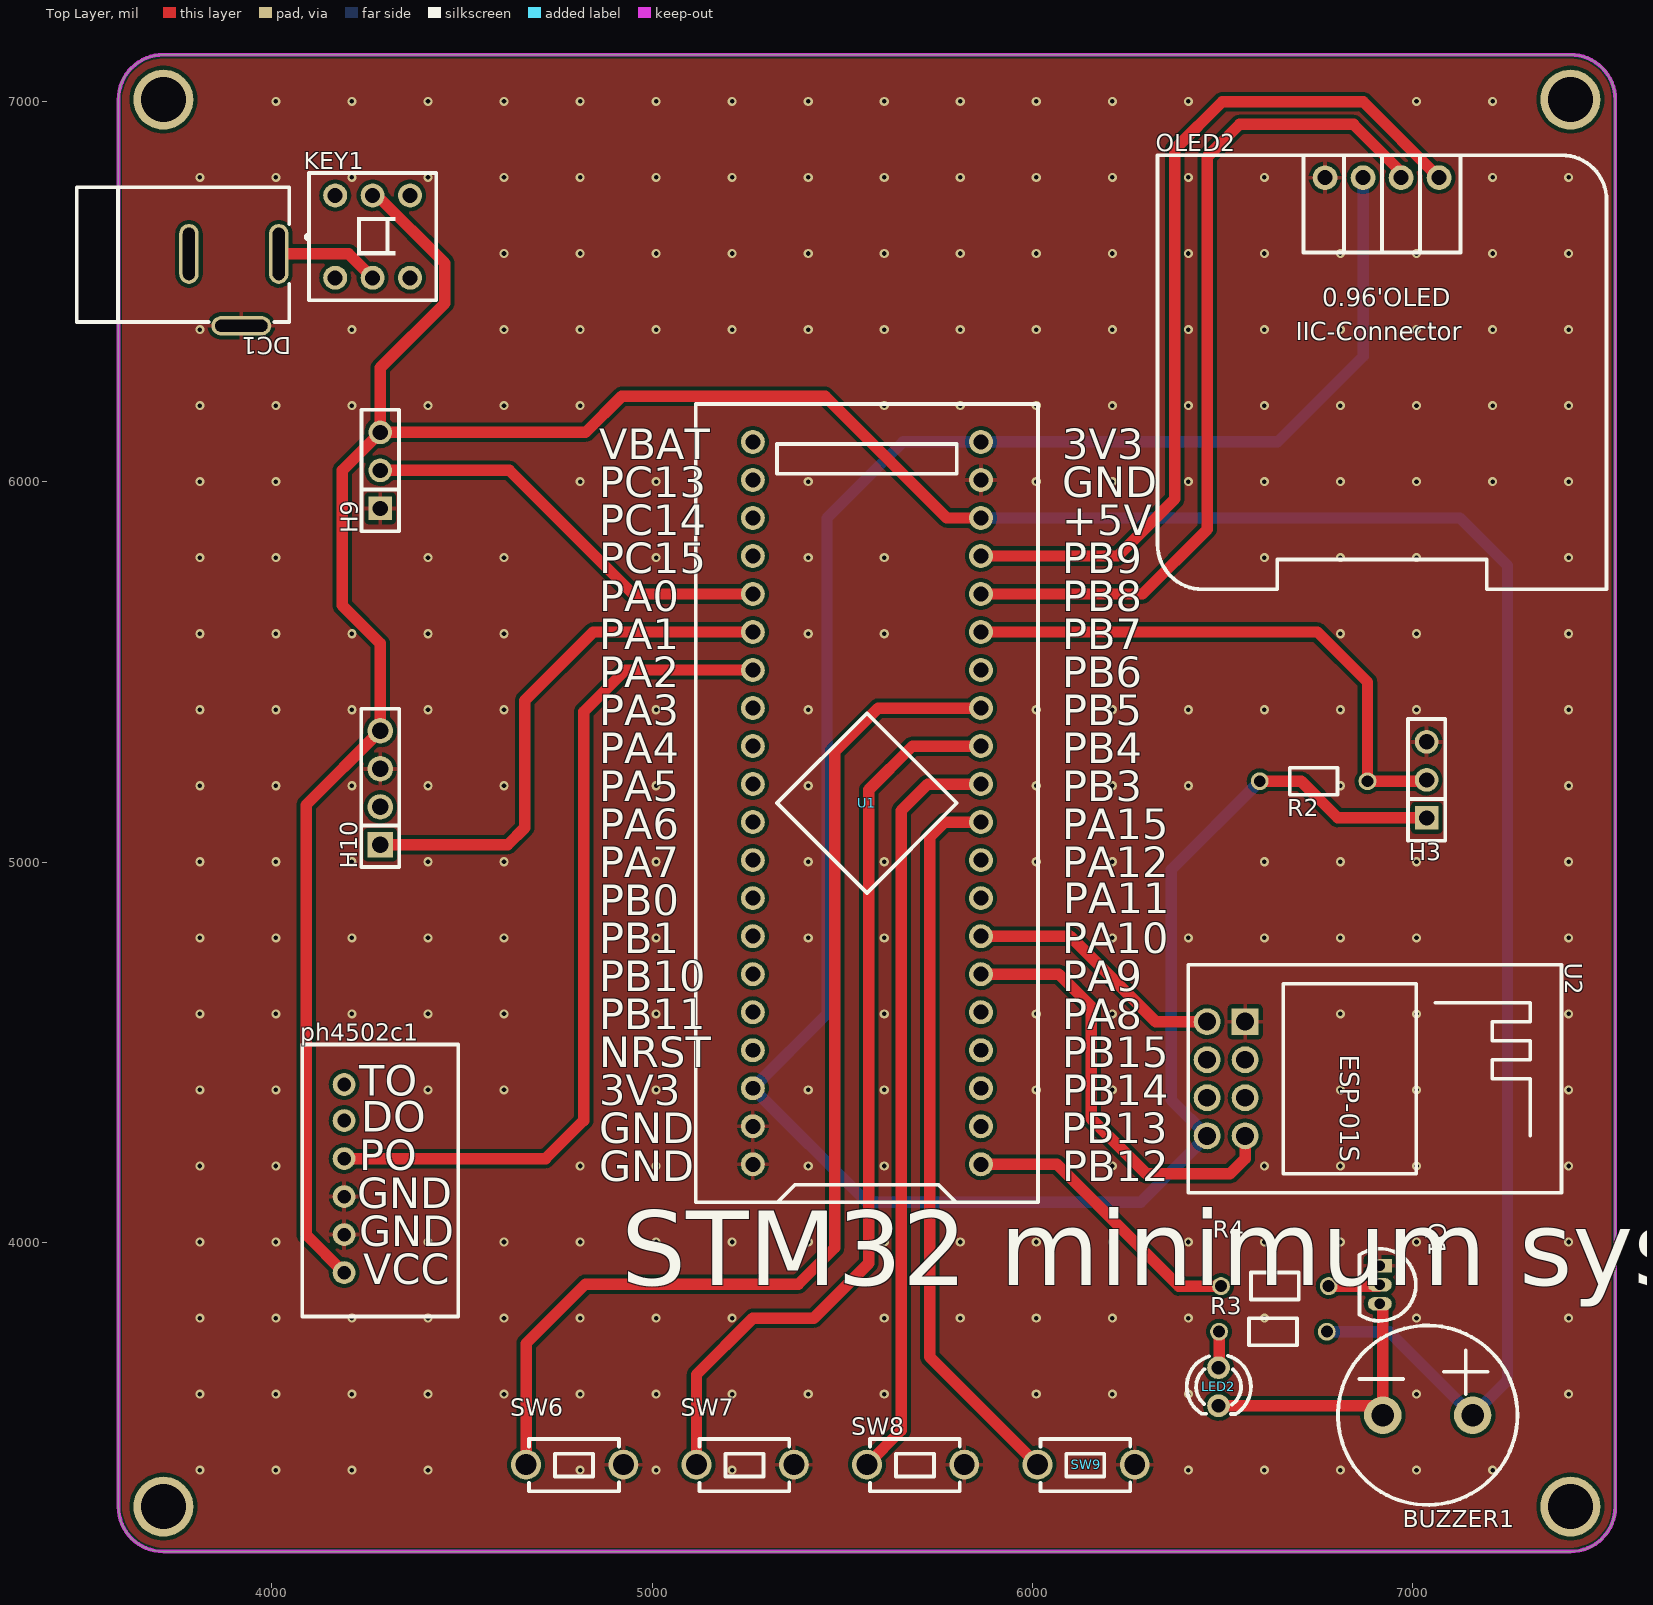
[diagram p0: Top Layer view]
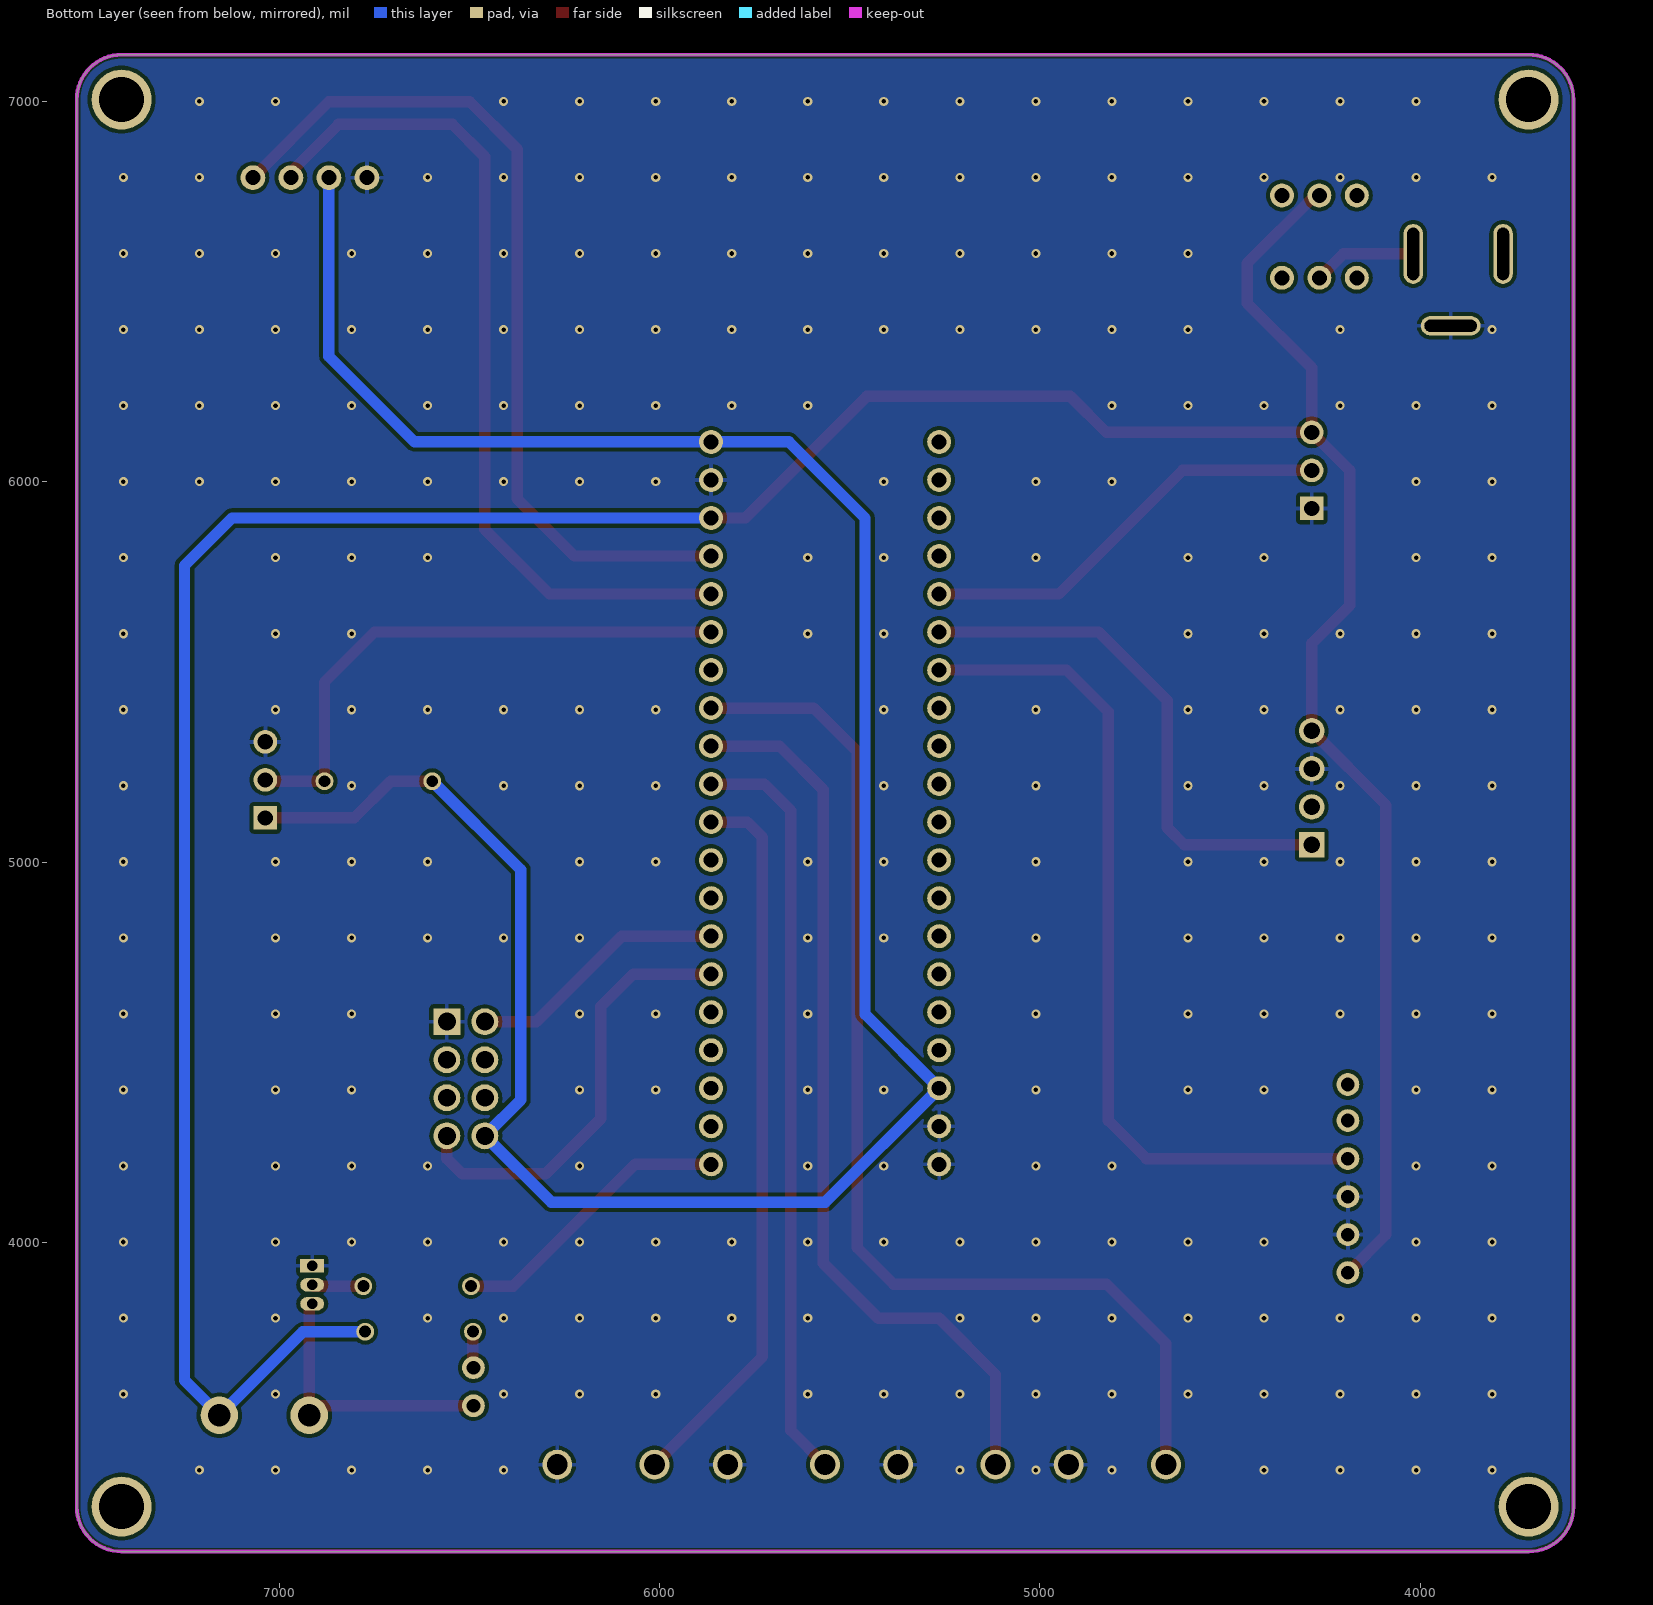
[diagram p1: Bottom Layer view, seen from below]
# Altium PCB MISC49912.pcbdoc
Units mil, origin at the board's own origin, x right, y up, seen from the top; angles counter-clockwise.
Board outline 3937.01 x 3937.01 mil, 2 copper layers (Top Layer, Bottom Layer), stack 62.206 mil thick; 19 components, 41 nets, 102 pads, 263 vias.

## Layer stack, top to bottom
Top Solder Mask Layer: solder mask 0.394, Dk 3.3
Top Layer: signal copper 1.379
Dielectric1: surface 59.449, FR4, Dk 4.5
Bottom Layer: signal copper 1.378
Bottom Solder Mask Layer: solder mask 0.394, Dk 3.3

## Board outline
3714.61,7123.5 ccw(c3714.61,7005.39) 3596.5,7005.39 3596.5,3304.61 ccw(c3714.61,3304.61) 3714.61,3186.5 7415.39,3186.5 ccw(c7415.39,3304.61) 7533.5,3304.61 7533.5,7005.39 ccw(c7415.39,7005.39) 7415.39,7123.5 3714.61,7123.5

## Design rules (kind name [scope] priority, off if disabled: settings)
BoardOutlineClearance copperThickness2oz_1 [All] p2 off: genericclearance=7.99 ignorepadtopadclearanceinfootprint=FALSE except(0: Arc-SplitContinuation Track-SplitContinuation SMDPad-SplitContinuation THPad-SplitContinuation Via-SplitContinuation Fill-SplitContinuation Region-SplitContinuation Poly-SplitContinuation Text-SplitContinuation Hole-SplitContinuation; 5.98: Arc-CutoutEdge Track-CutoutEdge SMDPad-CutoutEdge THPad-CutoutEdge Via-CutoutEdge Text-CutoutEdge; 6.9: Hole-OutlineEdge Hole-CutoutEdge; 10: Poly-OutlineEdge Poly-CutoutEdge; 11.81: Arc-OutlineEdge Track-OutlineEdge SMDPad-OutlineEdge THPad-OutlineEdge Via-OutlineEdge Fill-OutlineEdge Region-OutlineEdge Text-OutlineEdge Fill-CutoutEdge Region-CutoutEdge)
BoardOutlineClearance Plane_innerPlane_1 [All] p4 off: genericclearance=4.02 ignorepadtopadclearanceinfootprint=FALSE except(0: Arc-SplitContinuation Track-SplitContinuation SMDPad-SplitContinuation THPad-SplitContinuation Via-SplitContinuation Fill-SplitContinuation Region-SplitContinuation Poly-SplitContinuation Text-SplitContinuation Hole-SplitContinuation; 5.98: Arc-CutoutEdge Track-CutoutEdge SMDPad-CutoutEdge THPad-CutoutEdge Via-CutoutEdge Text-CutoutEdge; 6.9: Hole-OutlineEdge Hole-CutoutEdge; 10: Poly-OutlineEdge Poly-CutoutEdge; 11.81: Arc-OutlineEdge Track-OutlineEdge SMDPad-OutlineEdge THPad-OutlineEdge Via-OutlineEdge Fill-OutlineEdge Region-OutlineEdge Text-OutlineEdge Fill-CutoutEdge Region-CutoutEdge)
BoardOutlineClearance Copper_copperRegion_1 [All] p6 off: genericclearance=4.02 ignorepadtopadclearanceinfootprint=FALSE except(0: Arc-SplitContinuation Track-SplitContinuation SMDPad-SplitContinuation THPad-SplitContinuation Via-SplitContinuation Fill-SplitContinuation Region-SplitContinuation Poly-SplitContinuation Text-SplitContinuation Hole-SplitContinuation; 5.98: Arc-CutoutEdge Track-CutoutEdge SMDPad-CutoutEdge THPad-CutoutEdge Via-CutoutEdge Text-CutoutEdge; 6.9: Hole-OutlineEdge Hole-CutoutEdge; 10: Poly-OutlineEdge Poly-CutoutEdge; 11.81: Arc-OutlineEdge Track-OutlineEdge SMDPad-OutlineEdge THPad-OutlineEdge Via-OutlineEdge Fill-OutlineEdge Region-OutlineEdge Text-OutlineEdge Fill-CutoutEdge Region-CutoutEdge)
BoardOutlineClearance Copper_copperRegion_copperThickness1oz_1 [All] p8 off: genericclearance=4.02 ignorepadtopadclearanceinfootprint=FALSE except(0: Arc-SplitContinuation Track-SplitContinuation SMDPad-SplitContinuation THPad-SplitContinuation Via-SplitContinuation Fill-SplitContinuation Region-SplitContinuation Poly-SplitContinuation Text-SplitContinuation Hole-SplitContinuation; 5.98: Arc-CutoutEdge Track-CutoutEdge SMDPad-CutoutEdge THPad-CutoutEdge Via-CutoutEdge Text-CutoutEdge; 6.9: Hole-OutlineEdge Hole-CutoutEdge; 10: Poly-OutlineEdge Poly-CutoutEdge; 11.81: Arc-OutlineEdge Track-OutlineEdge SMDPad-OutlineEdge THPad-OutlineEdge Via-OutlineEdge Fill-OutlineEdge Region-OutlineEdge Text-OutlineEdge Fill-CutoutEdge Region-CutoutEdge)
BoardOutlineClearance Copper_copperRegion_Copper_copperRegion_1 [All] p10 off: genericclearance=4.02 ignorepadtopadclearanceinfootprint=FALSE except(0: Arc-SplitContinuation Track-SplitContinuation SMDPad-SplitContinuation THPad-SplitContinuation Via-SplitContinuation Fill-SplitContinuation Region-SplitContinuation Poly-SplitContinuation Text-SplitContinuation Hole-SplitContinuation; 5.98: Arc-CutoutEdge Track-CutoutEdge SMDPad-CutoutEdge THPad-CutoutEdge Via-CutoutEdge Text-CutoutEdge; 6.9: Hole-OutlineEdge Hole-CutoutEdge; 10: Poly-OutlineEdge Poly-CutoutEdge; 11.81: Arc-OutlineEdge Track-OutlineEdge SMDPad-OutlineEdge THPad-OutlineEdge Via-OutlineEdge Fill-OutlineEdge Region-OutlineEdge Text-OutlineEdge Fill-CutoutEdge Region-CutoutEdge)
BoardOutlineClearance copperThickness1oz_1 [All] p12: genericclearance=4.02 ignorepadtopadclearanceinfootprint=FALSE except(0: Arc-SplitContinuation Track-SplitContinuation SMDPad-SplitContinuation THPad-SplitContinuation Via-SplitContinuation Fill-SplitContinuation Region-SplitContinuation Poly-SplitContinuation Text-SplitContinuation Hole-SplitContinuation; 5.98: Arc-CutoutEdge Track-CutoutEdge SMDPad-CutoutEdge THPad-CutoutEdge Via-CutoutEdge Text-CutoutEdge; 6.9: Hole-OutlineEdge Hole-CutoutEdge; 10: Poly-OutlineEdge Poly-CutoutEdge; 11.81: Arc-OutlineEdge Track-OutlineEdge SMDPad-OutlineEdge THPad-OutlineEdge Via-OutlineEdge Fill-OutlineEdge Region-OutlineEdge Text-OutlineEdge Fill-CutoutEdge Region-CutoutEdge)
Clearance copperThickness2oz [All] p1 off: gap=7.99 ignorepadtopadclearanceinfootprint=FALSE except(5.98: SMDPad-Track SMDPad-SMDPad THPad-Track SMDPad-THPad THPad-THPad Track-Via SMDPad-Via THPad-Via Via-Via Fill-SMDPad Region-SMDPad Fill-THPad Region-THPad Fill-Via Region-Via Fill-Fill Fill-Region Region-Region Arc-Track Arc-SMDPad Arc-THPad Arc-Via Fill-Arc Region-Arc Arc-Arc Text-Track SMDPad-Text Text-THPad Text-Via Fill-Text Region-Text Arc-Text Text-Text; 6.9: Hole-Track Hole-SMDPad Hole-THPad Hole-Via Fill-Hole Region-Hole Hole-Arc Hole-Text; 10: Poly-Track Poly-SMDPad Poly-THPad Poly-Via Poly-Fill Poly-Region Poly-Poly Poly-Arc Poly-Text Poly-Hole; 11.81: Fill-Track Region-Track)
Clearance Plane_innerPlane [All] p3 off: gap=4.02 ignorepadtopadclearanceinfootprint=FALSE except(5.98: SMDPad-Track SMDPad-SMDPad THPad-Track SMDPad-THPad THPad-THPad Track-Via SMDPad-Via THPad-Via Via-Via Fill-SMDPad Region-SMDPad Fill-THPad Region-THPad Fill-Via Region-Via Fill-Fill Fill-Region Region-Region Arc-Track Arc-SMDPad Arc-THPad Arc-Via Fill-Arc Region-Arc Arc-Arc Text-Track SMDPad-Text Text-THPad Text-Via Fill-Text Region-Text Arc-Text Text-Text; 6.9: Hole-Track Hole-SMDPad Hole-THPad Hole-Via Fill-Hole Region-Hole Hole-Arc Hole-Text; 10: Poly-Track Poly-SMDPad Poly-THPad Poly-Via Poly-Fill Poly-Region Poly-Poly Poly-Arc Poly-Text Poly-Hole; 11.81: Fill-Track Region-Track)
Clearance Copper_copperRegion [All] p5 off: gap=4.02 ignorepadtopadclearanceinfootprint=FALSE except(5.98: SMDPad-Track SMDPad-SMDPad THPad-Track SMDPad-THPad THPad-THPad Track-Via SMDPad-Via THPad-Via Via-Via Fill-SMDPad Region-SMDPad Fill-THPad Region-THPad Fill-Via Region-Via Fill-Fill Fill-Region Region-Region Arc-Track Arc-SMDPad Arc-THPad Arc-Via Fill-Arc Region-Arc Arc-Arc Text-Track SMDPad-Text Text-THPad Text-Via Fill-Text Region-Text Arc-Text Text-Text; 6.9: Hole-Track Hole-SMDPad Hole-THPad Hole-Via Fill-Hole Region-Hole Hole-Arc Hole-Text; 10: Poly-Track Poly-SMDPad Poly-THPad Poly-Via Poly-Fill Poly-Region Poly-Poly Poly-Arc Poly-Text Poly-Hole; 11.81: Fill-Track Region-Track)
Clearance Copper_copperRegion_copperThickness1oz [All] p7 off: gap=4.02 ignorepadtopadclearanceinfootprint=FALSE except(5.98: SMDPad-Track SMDPad-SMDPad THPad-Track SMDPad-THPad THPad-THPad Track-Via SMDPad-Via THPad-Via Via-Via Fill-SMDPad Region-SMDPad Fill-THPad Region-THPad Fill-Via Region-Via Fill-Fill Fill-Region Region-Region Arc-Track Arc-SMDPad Arc-THPad Arc-Via Fill-Arc Region-Arc Arc-Arc Text-Track SMDPad-Text Text-THPad Text-Via Fill-Text Region-Text Arc-Text Text-Text; 6.9: Hole-Track Hole-SMDPad Hole-THPad Hole-Via Fill-Hole Region-Hole Hole-Arc Hole-Text; 10: Poly-Track Poly-SMDPad Poly-THPad Poly-Via Poly-Fill Poly-Region Poly-Poly Poly-Arc Poly-Text Poly-Hole; 11.81: Fill-Track Region-Track)
Clearance Copper_copperRegion_Copper_copperRegion [All] p9 off: gap=4.02 ignorepadtopadclearanceinfootprint=FALSE except(5.98: SMDPad-Track SMDPad-SMDPad THPad-Track SMDPad-THPad THPad-THPad Track-Via SMDPad-Via THPad-Via Via-Via Fill-SMDPad Region-SMDPad Fill-THPad Region-THPad Fill-Via Region-Via Fill-Fill Fill-Region Region-Region Arc-Track Arc-SMDPad Arc-THPad Arc-Via Fill-Arc Region-Arc Arc-Arc Text-Track SMDPad-Text Text-THPad Text-Via Fill-Text Region-Text Arc-Text Text-Text; 6.9: Hole-Track Hole-SMDPad Hole-THPad Hole-Via Fill-Hole Region-Hole Hole-Arc Hole-Text; 10: Poly-Track Poly-SMDPad Poly-THPad Poly-Via Poly-Fill Poly-Region Poly-Poly Poly-Arc Poly-Text Poly-Hole; 11.81: Fill-Track Region-Track)
Clearance copperThickness1oz [All] p11: gap=4.02 ignorepadtopadclearanceinfootprint=FALSE except(5.98: SMDPad-Track SMDPad-SMDPad THPad-Track SMDPad-THPad THPad-THPad Track-Via SMDPad-Via THPad-Via Via-Via Fill-SMDPad Region-SMDPad Fill-THPad Region-THPad Fill-Via Region-Via Fill-Fill Fill-Region Region-Region Arc-Track Arc-SMDPad Arc-THPad Arc-Via Fill-Arc Region-Arc Arc-Arc Text-Track SMDPad-Text Text-THPad Text-Via Fill-Text Region-Text Arc-Text Text-Text; 6.9: Hole-Track Hole-SMDPad Hole-THPad Hole-Via Fill-Hole Region-Hole Hole-Arc Hole-Text; 10: Poly-Track Poly-SMDPad Poly-THPad Poly-Via Poly-Fill Poly-Region Poly-Poly Poly-Arc Poly-Text Poly-Hole; 11.81: Fill-Track Region-Track)
DiffPairsRouting differentialPair [All] p1: maxlimit=6 minlimit=6 mostfreqgap=6 toplayer_minwidth=5 toplayer_prefwidth=10 toplayer_maxwidth=100 toplayer_mingap=6 toplayer_prefgap=6 toplayer_maxgap=6 bottomlayer_minwidth=5 bottomlayer_prefwidth=10 bottomlayer_maxwidth=100 bottomlayer_mingap=6 bottomlayer_prefgap=6 bottomlayer_maxgap=6 maxuncoupledlength=10
HoleToHoleClearance otherClearance [All] p1: gap=11.81 allowstackedmicrovias=TRUE
Length netLength [All] p1: minlimit=0 maxlimit=0
PasteMaskExpansion pasteMaskExpansion [All] p1: expansion=0
PlaneConnect innerPlane [All] p1: planeconnectstyle=Relief reliefexpansion=20 reliefentries=4 reliefconductorwidth=10 reliefairgap=10
PolygonConnect copperRegion_copperThickness1oz [All] p1 off: connectstyle=Relief reliefconductorwidth=10 reliefentries=4 polygonreliefangle="90 Angle" airgapwidth=10 via.connectstyle=Relief via.reliefconductorwidth=10 via.reliefentries=4 via.polygonreliefangle="90 Angle" via.airgapwidth=10
PolygonConnect copperRegion_Copper_copperRegion [All] p2 off: connectstyle=Relief reliefconductorwidth=10 reliefentries=4 polygonreliefangle="90 Angle" airgapwidth=10 via.connectstyle=Relief via.reliefconductorwidth=10 via.reliefentries=4 via.polygonreliefangle="90 Angle" via.airgapwidth=10
PolygonConnect copperRegion [All] p3: connectstyle=Relief reliefconductorwidth=10 reliefentries=4 polygonreliefangle="90 Angle" airgapwidth=10 via.connectstyle=Relief via.reliefconductorwidth=10 via.reliefentries=4 via.polygonreliefangle="90 Angle" via.airgapwidth=10
RoutingVias viaSize [All] p1: holewidth=12.01 width=24.02 viastyle="Through Hole" minholewidth=11.81 minwidth=19.68 maxholewidth=248.03 maxwidth=393.7
SolderMaskExpansion solderMaskExpansion [IsVia] p1: expansion=-1000 istentingtop=TRUE
SolderMaskExpansion solderMaskExpansion [All] p2: expansion=2 istentingtop=FALSE
Width copperThickness2oz_2 [All] p1 off: maxlimit=100 minlimit=8 preferedwidth=10
Width copperThickness1oz_2 [All] p2: maxlimit=100 minlimit=5 preferedwidth=10

## Components (designator, comment, footprint, x,y, rotation, side; value= is the part's Value field where it differs from the comment)
BUZZER1 "buzzer" BUZ-TH_BD12.0-P6.00-D0.9-RD 7040,3545 r0 top
DC1 "" DC-2.0 3895,6610 r180 top
H3 "" HDR-TH_3P-P2.54-V-F 7037.2,5216.04 r90 top
H9 "" HDR-TH_3P-P2.54-V-F 4285,6030 r90 top
H10 "" HDR-TH_4P-P2.54-V-F 4285,5195.08 r90 top
KEY1 "Non-self-locking switch 8.5×8.5 silent" SW-TH_6P-L8.5-W8.5-P2.54 4265,6645 r0 top
LED2 "" LED_TH-3mm 6490,3620 r270 top
OLED2 "" 0.96OLED_4P 6920,6800 r0 top
ph4502c1 "" PH4502C 4190,3920 r0 top
Q1 "" S8050_TO_92 6914,3888.14 r270 top
R2 "100" Res_1/8W 6740,5215 r180 top
R3 "10kΩ" Res_1/8W 6633.01,3762.14 r0 top
R4 "1kΩ" Res_1/8W 6638.01,3882.14 r0 top
SW6 "" Key_TH_3.5x6x4.3 4790,3415 r0 top
SW7 "" Key_TH_3.5x6x4.3 5238.33,3415 r0 top
SW8 "" Key_TH_3.5x6x4.3 5686.67,3415 r0 top
SW9 "" Key_TH_3.5x6x4.3 6135,3415 r0 top
U1 "STM32F103C8T6-Card" CONN-TH_L53.3-W22.9_STM32F103C8T6-CARD 5565,5155 r90 top
U2 "ESP-01S" WIFIM-TH_ESP-01S 6510,4430 r270 top

## Footprints (in the part's own frame and the unit in brackets; to place one, negate y for a bottom-side part, rotate by r counter-clockwise, add the part's x,y. Pads: shape width x height; smd on the part's side, far side on the other; paste and mask are expansions set on the pad)
0.96OLED_4P [mm]
  round 1.65 hole 1 copper offset 0,0: 1(-3.81,-0.001) 2(-1.27,0.002) 3(1.27,0.002) 4(3.81,0.002)
  silkscreen extent -15,-27.5 15,1.5
BUZ-TH_BD12.0-P6.00-D0.9-RD [mm]
  round 2.5 hole 1.5 paste+0 mask+0.05: 1(-3,0) 2(3,0)
  silkscreen extent -5.99,-5.99 5.99,5.99
CONN-TH_L53.3-W22.9_STM32F103C8T6-CARD [mm]
  round 1.6 hole 1: 1(-24.13,-7.62) 2(-21.59,-7.62) 3(-19.05,-7.62) 4(-16.51,-7.62) 5(-13.97,-7.62) 6(-11.43,-7.62) 7(-8.89,-7.62) 8(-6.35,-7.62) 9(-3.81,-7.62) 10(-1.27,-7.62) 11(1.27,-7.62) 12(3.81,-7.62) 13(6.35,-7.62) 14(8.89,-7.62) 15(11.43,-7.62) 16(13.97,-7.62) 17(16.51,-7.62) 18(19.05,-7.62) 19(21.59,-7.62) 20(24.13,-7.62) 21(24.13,7.62) 22(21.59,7.62) 23(19.05,7.62) 24(16.51,7.62) 25(13.97,7.62) 26(11.43,7.62) 27(8.89,7.62) 28(6.35,7.62) 29(3.81,7.62) 30(1.27,7.62) 31(-1.27,7.62) 32(-3.81,7.62) 33(-6.35,7.62) 34(-8.89,7.62) 35(-11.43,7.62) 36(-13.97,7.62) 37(-16.51,7.62) 38(-19.05,7.62) 39(-21.59,7.62) 40(-24.13,7.62)
  silkscreen extent -26.67,-11.43 26.67,11.43
DC-2.0 [mil]
  oval 157.5x51.2 hole 31.5 slot 137.8 at 0 deg paste+0 mask+2: 2(-24.7,199.5)
  oval 51.2x157.5 hole 31.5 slot 137.8 at 90 deg paste+0 mask+2: 3(113.1,10.5) 4(-123.1,10.5)
  silkscreen extent -151,-165 408,190
HDR-TH_3P-P2.54-V-F [mil]
  rect 62x62 hole 40.16: 1(-100,0)
  round 62 hole 40.16: 2(0,0) 3(100,0)
  silkscreen extent -160,-49 160,49
HDR-TH_4P-P2.54-V-F [mm]
  rect 1.7x1.7 hole 1.1: 1(-3.81,0)
  round 1.7 hole 1.1: 2(-1.27,0) 3(1.27,0) 4(3.81,0)
  silkscreen extent -5.29,-1.27 5.29,1.27
Key_TH_3.5x6x4.3 [mil]
  round 78.7 hole 55.1 paste+0 mask+2: A(-121.44,0) B(134.46,0)
  silkscreen extent -114,-70 123,68
LED_TH-3mm [mil]
  round 60 hole 36 paste+0 mask+2: 1(-50,0) 2(50,0)
  silkscreen extent -81,-84 72,85
PH4502C [mil]
  round 60 hole 36 paste+0 mask+2: 1(0,0) 2(0,100) 3(0,200) 4(0,300) 5(0,400) 6(0,495)
  silkscreen extent -110,-115 300,600
Res_1/8W [mil]
  round 47.2 hole 31.5 paste+0 mask+2: 1(-141.7,2.48) 2(141.7,2.48)
  silkscreen extent -63,-33 63,38
S8050_TO_92 [mil]
  rect 35.4x63 hole 27.6 paste+0 mask+2: 1(-50,0)
  oval 35.4x63 hole 27.6 paste+0 mask+2: 2(0,0) 3(50,0)
  silkscreen extent -95,-53 95,95
SW-TH_6P-L8.5-W8.5-P2.54 [mm]
  round 1.6 hole 1: 1(-2.5,-2.75) 2(0,-2.75) 3(2.5,-2.75) 4(-2.5,2.75) 5(0,2.75) 6(2.5,2.75)
  silkscreen extent -4.47,-4.25 4.25,4.25
WIFIM-TH_ESP-01S [mm]
  rect 1.8x1.8 hole 1.2: 1(-3.81,1.27)
  round 1.8 hole 1.2: 2(-1.27,1.27) 3(1.27,1.27) 4(3.81,1.27) 5(3.81,-1.27) 6(1.27,-1.27) 7(-1.27,-1.27) 8(-3.81,-1.27)
  silkscreen extent -7.62,-2.54 7.62,22.4

## Free pads (board coordinates)
  round 157.48 hole 118.11: 1(3714.61,7005.39) 1(3714.61,3304.61) 1(7415.39,7005.39) 1(7415.39,3304.61)

## Via types
v1: diameter 24.02, hole 12, Top Layer to Bottom Layer, 263 vias

## Nets (pads, with @x,y where several pads share a name; then routed paths per layer and width w, separated by ;. In a path a pad name is that pad's centre, name@x,y a point inside that pad or via, vN(x,y) a via of type N, cw(c..) or ccw(c..) an arc to the next point about the centre after c; other vN are vias at no path point)
$1N17250: DC1.4 KEY1.2 | length 272.9
  Top Layer w30: DC1.4 4202.23,6599.5 KEY1.2
$1N17253: LED2.1 R3.1 | length 95.2
  Top Layer w30: LED2.1 6491.31,3671.31 R3.1
$1N17254: BUZZER1.1 LED2.2 Q1.3 | length 738.7
  Top Layer w30: LED2.2 6896.89,3570 BUZZER1.1 6921.89,3830.26 Q1.3
$1N17255: Q1.2 R4.2 | length 135.8
  Top Layer w30: R4.2 6910.48,3884.62 Q1.2
+5V: BUZZER1.2 H9.3 H10.4 KEY1.5 ph4502c1.1 R3.2 U1.18 | length 9130.4
  Top Layer w30: ph4502c1.1 4090,4020 4090,5150.08 H10.4 4285,5575 4185,5675 4185,6030 H9.3 ; KEY1.5 4276.73,6753.27 4455,6575 4455,6470 4285,6300 H9.3 ; U1.18 5775,5905 5455,6225 4920,6225 4825,6130 H9.3
  Bottom Layer w30: U1.18 7125,5905 7250,5780 7250,3636.89 BUZZER1.2 6938.49,3764.62 R3.2
GND: DC1.2 H3.3 H9.1 H10.3 OLED2.1 ph4502c1.2 ph4502c1.3 Q1.1 SW6.B SW7.B SW8.B SW9.B U1.19 U1.39 U1.40 U2.1
  other v1: 3810.6,3400.6 4010.6,3400.6 4210.6,3400.6 4410.6,3400.6 4810.6,3400.6 5010.6,3400.6 5210.6,3400.6 6410.6,3400.6 6610.6,3400.6 6810.6,3400.6 7010.6,3400.6 7210.6,3400.6 3810.6,3600.6 4010.6,3600.6 4210.6,3600.6 4410.6,3600.6 4610.6,3600.6 4810.6,3600.6 5010.6,3600.6 5210.6,3600.6 5410.6,3600.6 5610.6,3600.6 6010.6,3600.6 6210.6,3600.6 6410.6,3600.6 7010.6,3600.6 7410.6,3600.6 3810.6,3800.6 4010.6,3800.6 4210.6,3800.6 4410.6,3800.6 4610.6,3800.6 4810.6,3800.6 5010.6,3800.6 5210.6,3800.6 5610.6,3800.6 5810.6,3800.6 6010.6,3800.6 6210.6,3800.6 6410.6,3800.6 6610.6,3800.6 7010.6,3800.6 7410.6,3800.6 3810.6,4000.6 4010.6,4000.6 4410.6,4000.6 4610.6,4000.6 4810.6,4000.6 5010.6,4000.6 5210.6,4000.6 5410.6,4000.6 5610.6,4000.6 5810.6,4000.6 6010.6,4000.6 6210.6,4000.6 6410.6,4000.6 6610.6,4000.6 6810.6,4000.6 7010.6,4000.6 7410.6,4000.6 3810.6,4200.6 4010.6,4200.6 4810.6,4200.6 5010.6,4200.6 5410.6,4200.6 5610.6,4200.6 6210.6,4200.6 6610.6,4200.6 6810.6,4200.6 7010.6,4200.6 7410.6,4200.6 3810.6,4400.6 4010.6,4400.6 4410.6,4400.6 4610.6,4400.6 5010.6,4400.6 5410.6,4400.6 5610.6,4400.6 6010.6,4400.6 6210.6,4400.6 6810.6,4400.6 7010.6,4400.6 7410.6,4400.6 3810.6,4600.6 4010.6,4600.6 4210.6,4600.6 4410.6,4600.6 4610.6,4600.6 5010.6,4600.6 5610.6,4600.6 6010.6,4600.6 6210.6,4600.6 6810.6,4600.6 7010.6,4600.6 7410.6,4600.6 3810.6,4800.6 4010.6,4800.6 4210.6,4800.6 4410.6,4800.6 4610.6,4800.6 5010.6,4800.6 5410.6,4800.6 5610.6,4800.6 6210.6,4800.6 6410.6,4800.6 6610.6,4800.6 6810.6,4800.6 7010.6,4800.6 7410.6,4800.6 3810.6,5000.6 4010.6,5000.6 4210.6,5000.6 4410.6,5000.6 4610.6,5000.6 5010.6,5000.6 5410.6,5000.6 5610.6,5000.6 6010.6,5000.6 6210.6,5000.6 6610.6,5000.6 6810.6,5000.6 7010.6,5000.6 7410.6,5000.6 3810.6,5200.6 4010.6,5200.6 4210.6,5200.6 4410.6,5200.6 4610.6,5200.6 5010.6,5200.6 5410.6,5200.6 6010.6,5200.6 6210.6,5200.6 6410.6,5200.6 6810.6,5200.6 7410.6,5200.6 3810.6,5400.6 4010.6,5400.6 4210.6,5400.6 4410.6,5400.6 4610.6,5400.6 5010.6,5400.6 5410.6,5400.6 6010.6,5400.6 6210.6,5400.6 6410.6,5400.6 6610.6,5400.6 6810.6,5400.6 7010.6,5400.6 7410.6,5400.6 3810.6,5600.6 4010.6,5600.6 4210.6,5600.6 4410.6,5600.6 4610.6,5600.6 5410.6,5600.6 5610.6,5600.6 6810.6,5600.6 7010.6,5600.6 7410.6,5600.6 3810.6,5800.6 4010.6,5800.6 4410.6,5800.6 4610.6,5800.6 5010.6,5800.6 5410.6,5800.6 5610.6,5800.6 6610.6,5800.6 6810.6,5800.6 7010.6,5800.6 7410.6,5800.6 3810.6,6000.6 4010.6,6000.6 4810.6,6000.6 5010.6,6000.6 5410.6,6000.6 6010.6,6000.6 6210.6,6000.6 6410.6,6000.6 6610.6,6000.6 6810.6,6000.6 7010.6,6000.6 7210.6,6000.6 7410.6,6000.6 3810.6,6200.6 4010.6,6200.6 4210.6,6200.6 4410.6,6200.6 4610.6,6200.6 4810.6,6200.6 5610.6,6200.6 5810.6,6200.6 6010.6,6200.6 6210.6,6200.6 6410.6,6200.6 6610.6,6200.6 6810.6,6200.6 7010.6,6200.6 7210.6,6200.6 7410.6,6200.6 3810.6,6400.6 4210.6,6400.6 4610.6,6400.6 4810.6,6400.6 5010.6,6400.6 5210.6,6400.6 5410.6,6400.6 5610.6,6400.6 5810.6,6400.6 6010.6,6400.6 6210.6,6400.6 6410.6,6400.6 6610.6,6400.6 6810.6,6400.6 7010.6,6400.6 7210.6,6400.6 7410.6,6400.6 4610.6,6600.6 4810.6,6600.6 5010.6,6600.6 5210.6,6600.6 5410.6,6600.6 5610.6,6600.6 5810.6,6600.6 6010.6,6600.6 6210.6,6600.6 6410.6,6600.6 6610.6,6600.6 6810.6,6600.6 7010.6,6600.6 7210.6,6600.6 7410.6,6600.6 3810.6,6800.6 4010.6,6800.6 4210.6,6800.6 4410.6,6800.6 4610.6,6800.6 4810.6,6800.6 5010.6,6800.6 5210.6,6800.6 5410.6,6800.6 5610.6,6800.6 5810.6,6800.6 6010.6,6800.6 6210.6,6800.6 6410.6,6800.6 6610.6,6800.6 7210.6,6800.6 7410.6,6800.6 4010.6,7000.6 4210.6,7000.6 4410.6,7000.6 4610.6,7000.6 4810.6,7000.6 5010.6,7000.6 5210.6,7000.6 5410.6,7000.6 5610.6,7000.6 5810.6,7000.6 6010.6,7000.6 6210.6,7000.6 6410.6,7000.6 7010.6,7000.6 7210.6,7000.6
NRST: U1.37
PA0: H9.2 U1.25 | length 1114.6
  Top Layer w30: H9.2 4625,6030 4950,5705 U1.25
PA1: H10.1 U1.26 | length 1408.2
  Top Layer w30: H10.1 4620.08,5045.08 4665,5090 4665,5425 4845,5605 U1.26
PA2: ph4502c1.4 U1.27 | length 2237
  Top Layer w30: ph4502c1.4 4720,4220 4820,4320 4820,5395 4930,5505 U1.27
PA3: U1.28
PA4: U1.29
PA5: U1.30
PA6: U1.31
PA7: U1.32
PA8: U1.5
PA9: U1.6 U2.4 | length 1161.8
  Top Layer w30: U1.6 6070,4705 6155,4620 6155,4325 6300,4180 6520,4180 6560,4220 U2.4
PA10: U1.7 U2.8 | length 688.2
  Top Layer w30: U1.7 6100,4805 6325,4580 U2.8
PA11: U1.8
PA12: U1.9
PA15: SW9.A U1.10 | length 1919
  Top Layer w30: U1.10 5770,5105 5730,5065 5730,3698.56 SW9.A
PB0: U1.33
PB1: U1.34
PB3: SW8.A U1.11 | length 1996.2
  Top Layer w30: SW8.A 5655,3504.77 5655,5135 5725,5205 U1.11
PB4: SW7.A U1.12 | length 2399
  Top Layer w30: SW7.A 5116.89,3651.89 5265,3800 5425,3800 5570,3945 5570,5190 5685,5305 U1.12
PB5: SW6.A U1.13 | length 2971.8
  Top Layer w30: SW6.A 4668.56,3733.56 4825,3890 5385,3890 5480,3985 5480,5290 5595,5405 U1.13
PB6: U1.14
PB7: H3.2 R2.1 U1.15 | length 1489
  Top Layer w30: U1.15 6750,5605 6881.7,5473.3 R2.1 7033.68,5212.52 H3.2
PB8: OLED2.3 U1.16 | length 2257.4
  Top Layer w30: U1.16 6290,5705 6460,5875 6460,6855 6545,6940 6845,6940 6970,6815 OLED2.3@6970,6800.05
PB9: OLED2.4 U1.17 | length 2321.7
  Top Layer w30: U1.17 6225,5805 6375,5955 6375,6875 6500,7000 6870.05,7000 OLED2.4@7070,6800.05
PB10: U1.35
PB11: U1.36
PB12: R4.1 U1.1 | length 764
  Top Layer w30: U1.1 6065,4205 6385.38,3884.62 R4.1
PB13: U1.2
PB14: U1.3
PB15: U1.4
PC13: U1.22
PC14: U1.23
PC15: U1.24
VBAT: U1.21
VCC: H3.1 OLED2.2 R2.2 U1.20 U1.38 U2.5 | length 6576
  Top Layer w30: R2.2 6707.48,5212.52 6803.96,5116.04 H3.1
  Bottom Layer w30: R2.2 6365,4979.22 6365,4375 U2.5 6285,4105 5565,4105 U1.38 5460,4600 5460,5905 5660,6105 U1.20 6645,6105 6870,6330 OLED2.2@6870,6800.05
pads on no net: DC1.3 H10.2 KEY1.1 KEY1.3 KEY1.4 KEY1.6 ph4502c1.5 ph4502c1.6 U2.2 U2.3 U2.6 U2.7

## Polygon pours and split planes (outlines as drawn)
GND on Bottom Layer (solid, remove dead copper, pour order 2): 3525,7245 3525,3080 7700,3080 7700,7245
GND on Top Layer (solid, remove dead copper, pour order 2): 3000,7415 3000,3000 7930,3000 7930,7415

## Keep-outs
Board Outline Layer:
  the board outline again, w10

## Silkscreen, mask and mechanical layers (free items; w line width, h text height)
Top Silkscreen Layer:
  text "VBAT" at 4860.95,6060 h80
  text "3V3" at 6079.16,6060 h80
  text "PC13" at 4860.95,5960 h80
  text "GND" at 6079.16,5960 h80
  text "PC14" at 4860.95,5860 h80
  text "+5V" at 6079.16,5860 h80
  text "PC15" at 4860.95,5760 h80
  text "PB9" at 6079.16,5760 h80
  text "PA0" at 4860.95,5660 h80
  text "PB8" at 6079.16,5660 h80
  text "PA1" at 4860.95,5560 h80
  text "PB7" at 6079.16,5560 h80
  text "PA2" at 4860.95,5460 h80
  text "PB6" at 6079.16,5460 h80
  text "PA3" at 4860.95,5360 h80
  text "PB5" at 6079.16,5360 h80
  text "PA4" at 4860.95,5260 h80
  text "PB4" at 6079.16,5260 h80
  text "PA5" at 4860.95,5160 h80
  text "PB3" at 6079.16,5160 h80
  text "PA6" at 4860.95,5060 h80
  text "PA15" at 6079.16,5060 h80
  text "PA7" at 4860.95,4960 h80
  text "PA12" at 6079.16,4960 h80
  text "PA11" at 6080.95,4865 h80
  text "PB0" at 4860.95,4860 h80
  text "PB1" at 4860.95,4760 h80
  text "PA10" at 6079.16,4760 h80
  text "PB10" at 4860.95,4660 h80
  text "PA9" at 6079.16,4660 h80
  text "PB11" at 4860.95,4560 h80
  text "PA8" at 6079.16,4560 h80
  text "NRST" at 4860.95,4460 h80
  text "PB15" at 6079.16,4460 h80
  text "3V3" at 4860.95,4360 h80
  text "PB14" at 6079.16,4360 h80
  text "GND" at 4860.95,4260 h80
  text "PB13" at 6075.95,4260 h80
  text "GND" at 4860.95,4160 h80
  text "PB12" at 6079.16,4160 h80
  text "STM32 minimum system" at 4919.45,3886.57 h196.85